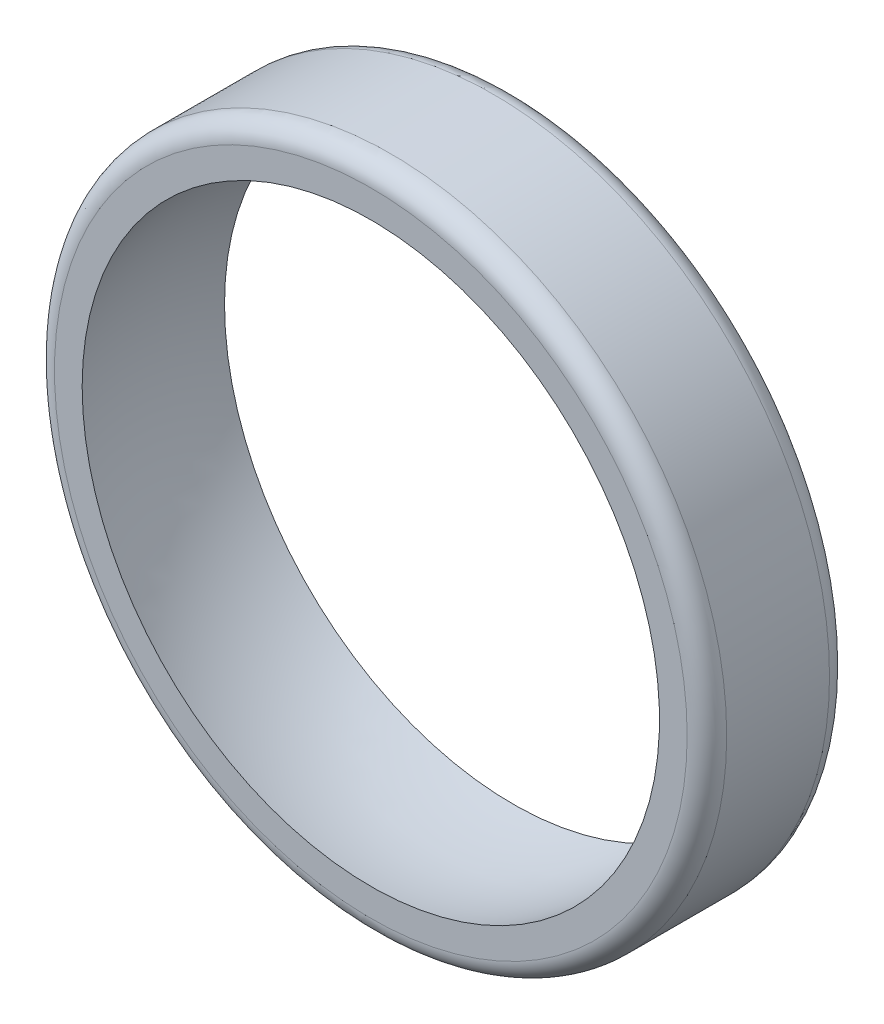
from build123d import *

# Parameters (mm, degrees)
SKETCH1_R           = 42.5
SKETCH1_R_2         = 36.5
BOSS_EXTRUDE1_DEPTH = 9
FILLET1_R           = 2.5


with BuildPart() as part:
    # Sketch1 → Boss-Extrude1 (new, symmetric)
    with BuildSketch(Plane.XY):
        Circle(SKETCH1_R)
        Circle(SKETCH1_R_2, mode=Mode.SUBTRACT)
    extrude(amount=BOSS_EXTRUDE1_DEPTH, both=True)

    # Sketch2 → Cut-Revolve1 (revolve, cut)
    with BuildSketch(Plane(origin=(0, 0, 0), x_dir=(1, 0, 0), z_dir=(0, 1, 0)), mode=Mode.PRIVATE) as cut_revolve1_sk:
        with BuildLine():
            Line((36.5, 9), (36.5, -9))
            ThreePointArc((36.5, -9), (37.40918463, 0), (36.5, 9))
        make_face()
    revolve(cut_revolve1_sk.sketch.rotate(Axis((0, 0, 0), (0, 0, 1)), 180), axis=Axis((0, 0, 0), (0, 0, 1)), mode=Mode.SUBTRACT)

    # Fillet1
    fillet1_edges = [part.edges().sort_by_distance(p)[0] for p in [
        (-42.5, 0, -9),
        (-42.5, 0, 9),
    ]]
    fillet(fillet1_edges, radius=FILLET1_R)


solid = part.part
